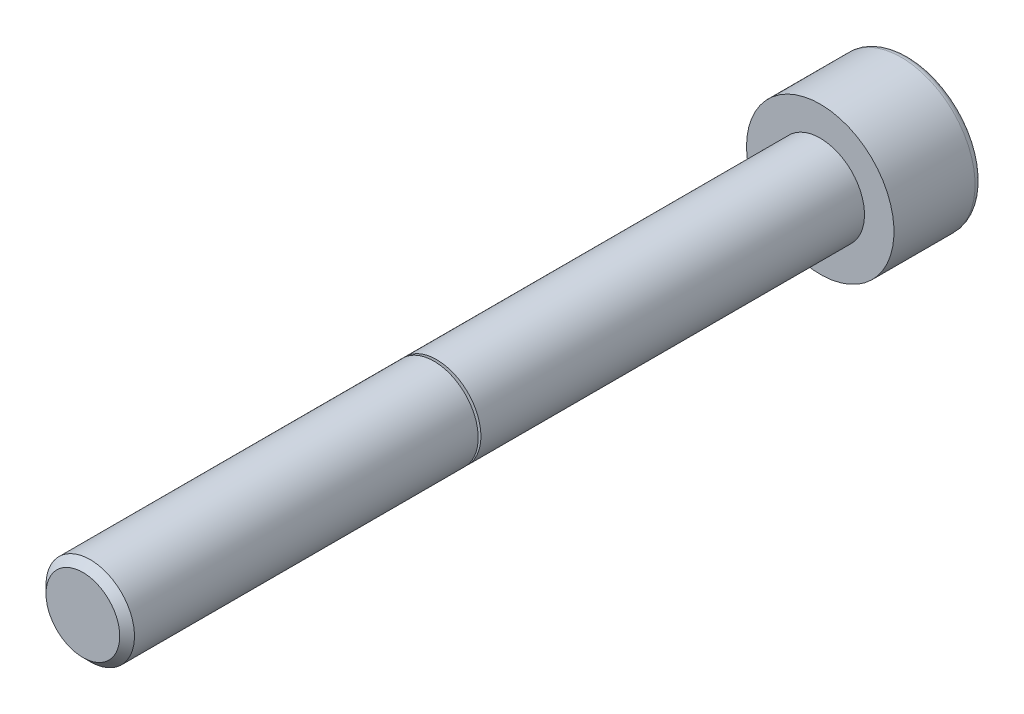
SolidWorks part; units mm, degrees
ref_plane "Front" through (0, 0, 0) normal (0, 0, 1) x (1, 0, 0)
ref_plane "Top" through (0, 0, 0) normal (0, 1, 0) x (1, 0, 0)
ref_plane "Right" through (0, 0, 0) normal (1, 0, 0) x (0, 0, -1)
sketch "Logo3_Revol_Axis" plane through (0, 0, 0) normal (0, 1, 0) x (1, 0, 0)
  line L0 (0, -43.5172) -> (0, 43.5172) construction
sketch "Logo3_bib1" plane through (0, 0, 0) normal (0, -1, 0) x (-1, 0, 0)
  line L0 (0, -50) -> (0, 6)
  line L1 (0, 6) -> (4.5, 6)
  line L2 (5, 5.5) -> (5, 0)
  line L3 (5, 0) -> (3, 0)
  line L4 (3, 0) -> (3, -26.01)
  line L5 (3, -49.5) -> (2.5, -50)
  line L6 (2.5, -50) -> (0, -50)
  line L7 (3, -26.01) -> (2.6134, -26.01)
  line L8 (2.6066, -26.0488) -> (3, -26.192)
  line L9 (3, -26.192) -> (3, -49.5)
  line L10 (0, 10.5852) -> (0, -63.2873) construction
  arc A0 (4.5, 6) -> (5, 5.5) centre (4.5, 5.5) cw
  arc A1 (2.6134, -26.01) -> (2.6066, -26.0488) centre (2.6134, -26.03) ccw
  point P17 (2.5, -26.01)
revolve "Revolve1" add sketch "Logo3_bib1" angle 360 about L10
cosmetic thread "Cosmetic Thread1" parameters "D2"=5
sketch "Logo3_bib2" plane through (0, 0, -6) normal (0, 0, -1) x (1, 0, 0)
  line L1 (2.8868, 0) -> (1.4434, 2.5)
  line L2 (1.4434, 2.5) -> (-1.4434, 2.5)
  line L3 (-1.4434, 2.5) -> (-2.8868, 0)
  line L4 (-2.8868, 0) -> (-1.4434, -2.5)
  line L5 (-1.4434, -2.5) -> (1.4434, -2.5)
  line L6 (1.4434, -2.5) -> (2.8868, 0)
  circle A0 centre (0, 0) radius 2.5 construction
extrude "Cut-Extrude1" cut sketch "Logo3_bib2" against normal blind 2.5
equation "\"DIA2@XZQB7_bib1\" = \"XZQB7_d1-pas@XZQB7_bib1\""
equation "\"LGT1@XZQB7_bib1\" = \"XZQB7_d1@XZQB7_bib1\""
equation "\"D1@Cut-Extrude1\" = \"XZQB7_c1@XZQB7_bib2\"/2."
equation "\"D2@Cosmetic Thread1\" = \"XZQB7_d1-pas@XZQB7_bib1\""
